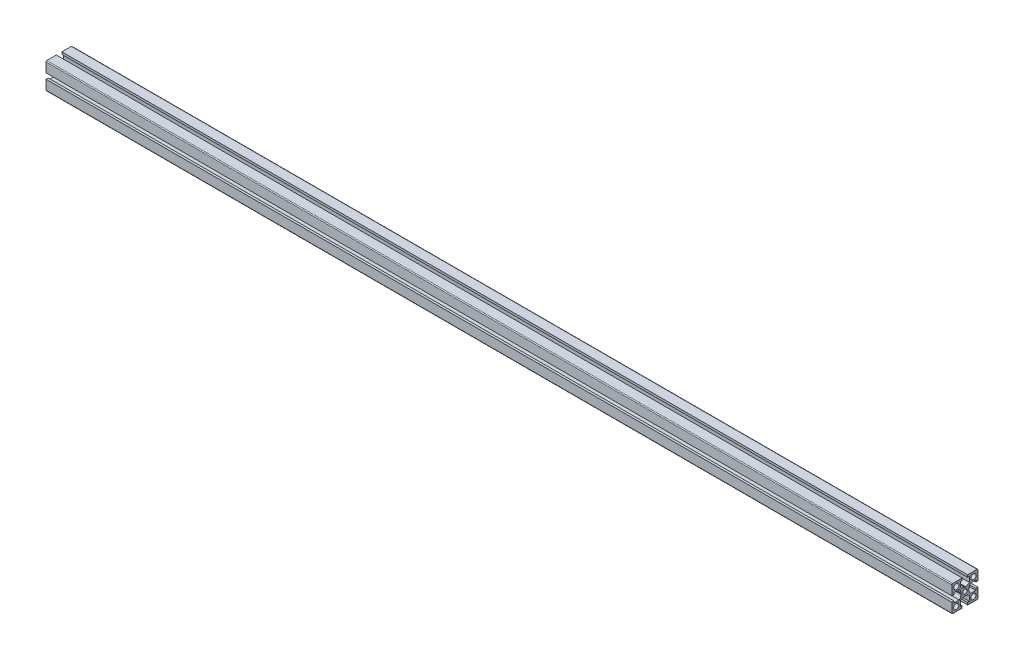
from build123d import *

# Parameters (mm, degrees)
SKETCH_11_R         = 3
SKETCH_11_R_2       = 2.5
F_0_GY_3030_1_DEPTH = 1040


with BuildPart() as part:
    # 草图11 → 0国耀铝型材 GY-3030国标铝型材(1) (new body)
    with BuildSketch(Plane(origin=(0, 0, 0), x_dir=(0, 0, -1), z_dir=(1, 0, 0))):
        with BuildLine():
            Line((-14, -15), (-3.15, -15))
            Line((-3.15, -15), (-3.15, -12.5))
            Line((-3.15, -12.5), (-5.15, -12.5))
            Line((-5.15, -12.5), (-5.15, -6.5))
            ThreePointArc((-5.15, -6.5), (-3.019390742, -5.122695475), (-0.555, -4.52))
            Line((-0.555, -4.52), (0, -4.2))
            Line((0, -4.2), (0.555, -4.52))
            ThreePointArc((0.555, -4.52), (3.019390742, -5.122695475), (5.15, -6.5))
            Line((5.15, -6.5), (5.15, -12.5))
            Line((5.15, -12.5), (3.15, -12.5))
            Line((3.15, -12.5), (3.15, -15))
            Line((3.15, -15), (14, -15))
            ThreePointArc((14, -15), (14.707106781, -14.707106781), (15, -14))
            Line((15, -14), (15, -3.15))
            Line((15, -3.15), (12.5, -3.15))
            Line((12.5, -3.15), (12.5, -5.15))
            Line((12.5, -5.15), (6.5, -5.15))
            ThreePointArc((6.5, -5.15), (5.12253592, -3.018923167), (4.52, -0.554))
            Line((4.52, -0.554), (4.2, 0))
            Line((4.2, 0), (4.52, 0.555))
            ThreePointArc((4.52, 0.555), (5.122695475, 3.019390742), (6.5, 5.15))
            Line((6.5, 5.15), (12.5, 5.15))
            Line((12.5, 5.15), (12.5, 3.15))
            Line((12.5, 3.15), (15, 3.15))
            Line((15, 3.15), (15, 14))
            ThreePointArc((15, 14), (14.707106781, 14.707106781), (14, 15))
            Line((14, 15), (3.15, 15))
            Line((3.15, 15), (3.15, 12.5))
            Line((3.15, 12.5), (5.15, 12.5))
            Line((5.15, 12.5), (5.15, 6.5))
            ThreePointArc((5.15, 6.5), (3.019292492, 5.123227892), (0.555, 4.521))
            Line((0.555, 4.521), (0, 4.2))
            Line((0, 4.2), (-0.555, 4.521))
            ThreePointArc((-0.555, 4.521), (-3.019292492, 5.123227892), (-5.15, 6.5))
            Line((-5.15, 6.5), (-5.15, 12.5))
            Line((-5.15, 12.5), (-3.15, 12.5))
            Line((-3.15, 12.5), (-3.15, 15))
            Line((-3.15, 15), (-14, 15))
            ThreePointArc((-14, 15), (-14.707106781, 14.707106781), (-15, 14))
            Line((-15, 14), (-15, 3.15))
            Line((-15, 3.15), (-12.5, 3.15))
            Line((-12.5, 3.15), (-12.5, 5.15))
            Line((-12.5, 5.15), (-6.5, 5.15))
            ThreePointArc((-6.5, 5.15), (-5.122695475, 3.019390742), (-4.52, 0.555))
            Line((-4.52, 0.555), (-4.2, 0))
            Line((-4.2, 0), (-4.52, -0.554))
            ThreePointArc((-4.52, -0.554), (-5.12253592, -3.018923167), (-6.5, -5.15))
            Line((-6.5, -5.15), (-12.5, -5.15))
            Line((-12.5, -5.15), (-12.5, -3.15))
            Line((-12.5, -3.15), (-15, -3.15))
            Line((-15, -3.15), (-15, -14))
            ThreePointArc((-15, -14), (-14.707106781, -14.707106781), (-14, -15))
        make_face()
        with Locations((9.8, 9.9)):
            Circle(SKETCH_11_R, mode=Mode.SUBTRACT)
        with Locations((9.8, -9.9)):
            Circle(SKETCH_11_R, mode=Mode.SUBTRACT)
        Circle(SKETCH_11_R_2, mode=Mode.SUBTRACT)
        with Locations((-9.8, 9.9)):
            Circle(SKETCH_11_R, mode=Mode.SUBTRACT)
        with Locations((-10, -9.9)):
            Circle(SKETCH_11_R, mode=Mode.SUBTRACT)
    extrude(amount=F_0_GY_3030_1_DEPTH)


solid = part.part
